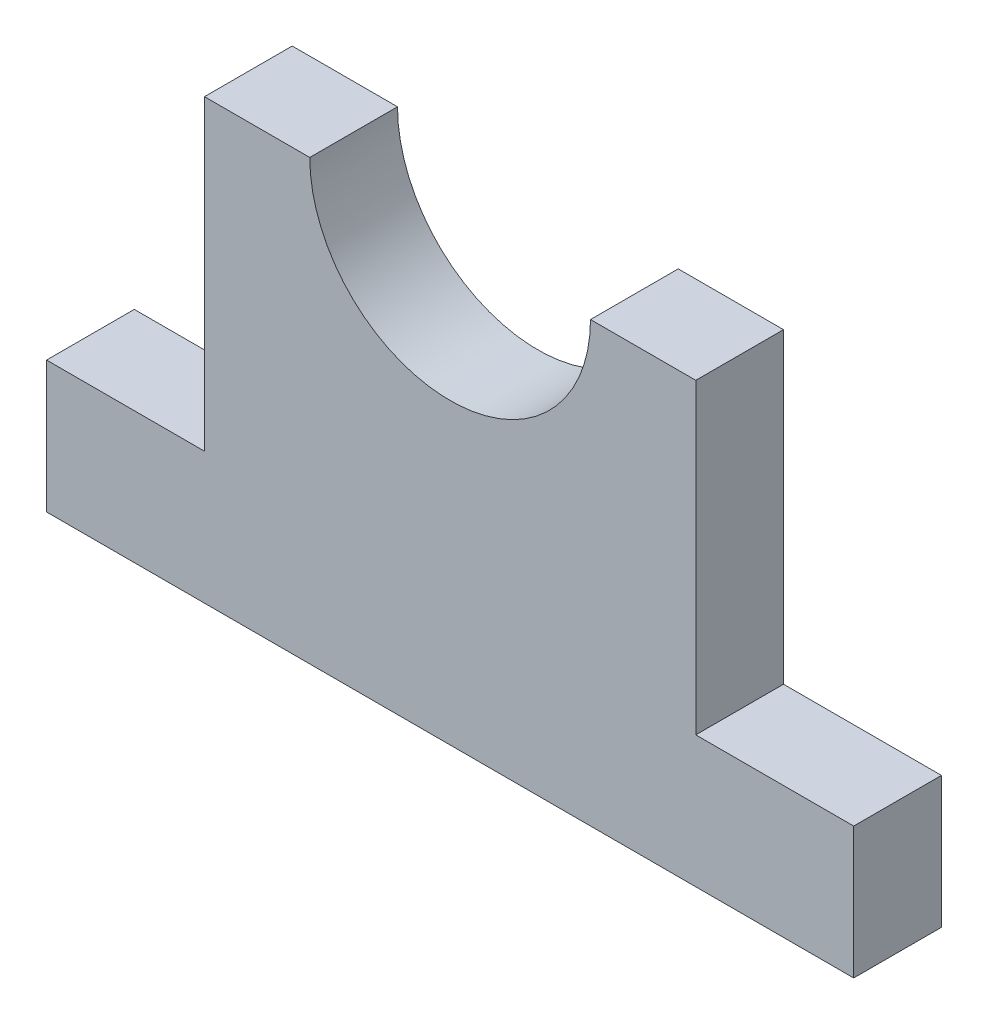
from build123d import *

# Parameters (mm, degrees)
BOSS_EXTRUDE1_DEPTH = 10


with BuildPart() as part:
    # Sketch1 → Boss-Extrude1 (new body)
    with BuildSketch(Plane.XY):
        with BuildLine():
            Line((-16, 50), (-28, 50))
            Line((-28, 50), (-28, 15))
            Line((-28, 15), (-46, 15))
            Line((-46, 15), (-46, 0))
            Line((-46, 0), (46, 0))
            Line((46, 0), (46, 15))
            Line((46, 15), (28, 15))
            Line((28, 15), (28, 50))
            Line((28, 50), (16, 50))
            ThreePointArc((16, 50), (0, 34), (-16, 50))
        make_face()
    extrude(amount=BOSS_EXTRUDE1_DEPTH)


solid = part.part
